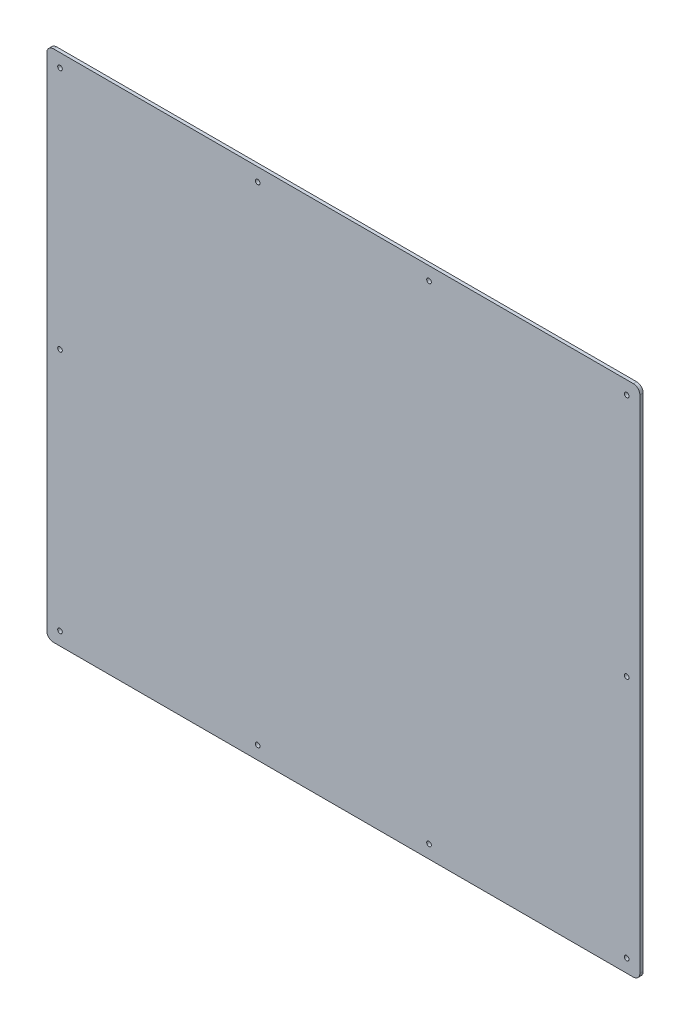
SolidWorks part; units mm, degrees
material "PMMA（透明）"
ref_plane "前视基准面" through (0, 0, 0) normal (0, 0, 1) x (1, 0, 0)
ref_plane "上视基准面" through (0, 0, 0) normal (0, 1, 0) x (1, 0, 0)
ref_plane "右视基准面" through (0, 0, 0) normal (1, 0, 0) x (0, 0, -1)
sketch "草图1" plane through (0, 0, 0) normal (0, 0, 1) x (1, 0, 0)
  line L1 (-450, -390) -> (450, -390)
  line L2 (-450, -390) -> (-450, 390)
  line L3 (-450, 390) -> (450, 390)
  line L4 (450, -390) -> (450, 390)
  line L5 (-450, -390) -> (450, 390) construction
  line L6 (-450, 390) -> (450, -390) construction
  point P0 (0, 0)
  dimension "D1" = 900
  dimension "D2" = 780
extrude "凸台-拉伸1" add sketch "草图1" along normal blind 5
hole_wizard "Ø7.0 (7) 直径孔1" positions "草图2" profile "草图3" hole size "Ø7.0" standard "ISO"
sketch "草图2" plane through (0, 0, 5) normal (0, 0, 1) x (1, 0, 0)
  line L0 (-450, 0) -> (450, 0) construction
  line L1 (-450, 390) -> (-450, -390) construction
  line L2 (450, -390) -> (450, 390) construction
  line L4 (0, 390) -> (0, -390) construction
  line L5 (450, 390) -> (-450, 390) construction
  line L6 (-450, -390) -> (450, -390) construction
  point P0 (-430, 370)
  point P2 (430, 370)
  point P21 (430, -370)
  point P22 (-430, -370)
  point P23 (-430, 0)
  point P27 (430, 0)
  point P28 (-130, 370)
  point P30 (130, 370)
  point P32 (-130, -370)
  point P34 (130, -370)
  dimension "D1" = 20
  dimension "D2" = 20
  dimension "D3" = 300
  dimension "D4" = 300
  dimension "D5" = 300
  dimension "D6" = 300
sketch "草图3" plane through (-430, 370, 5) normal (1, 0, 0) x (0, -1, 0)
  line L0 (0, 0) -> (0, 29.853)
  line L1 (0, 29.853) -> (3.5, 27.75)
  line L2 (3.5, 27.75) -> (3.5, 0)
  line L5 (3.5, 0) -> (0, 0)
  line L10 (0, 29.853) -> (-3.5, 27.75) construction
  line L11 (0, -6.35) -> (0, 107.95) construction
  dimension "孔直径" = 7
  dimension "孔深度" = 27.75
  dimension "导头角度" = 118
fillet "圆角1" radius 10 4 edges at (-450, -390, 2.5) (450, -390, 2.5) (450, 390, 2.5) (-450, 390, 2.5)
